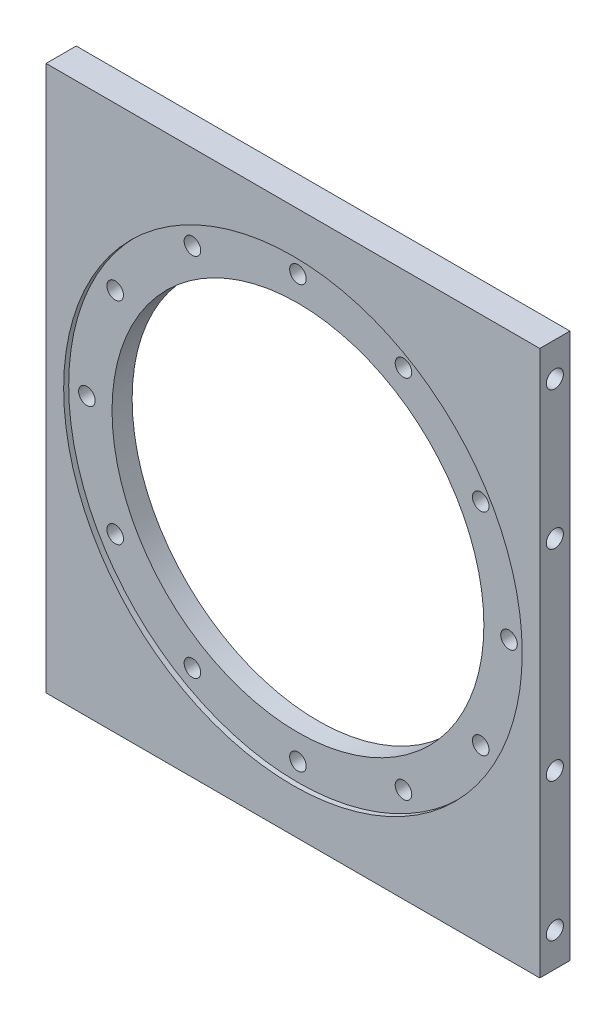
SolidWorks part; units mm, degrees
material "Q235A"
ref_plane "前视基准面" through (0, 0, 0) normal (0, 0, 1) x (1, 0, 0)
ref_plane "上视基准面" through (0, 0, 0) normal (0, 1, 0) x (1, 0, 0)
ref_plane "右视基准面" through (0, 0, 0) normal (1, 0, 0) x (0, 0, -1)
sketch "草图1" plane through (0, 0, 0) normal (0, 0, 1) x (1, 0, 0)
  line L1 (-98.25, -108.5) -> (98.25, -108.5)
  line L2 (-98.25, -108.5) -> (-98.25, 108.5)
  line L3 (-98.25, 108.5) -> (98.25, 108.5)
  line L4 (98.25, -108.5) -> (98.25, 108.5)
  line L5 (-98.25, -108.5) -> (98.25, 108.5) construction
  line L6 (-98.25, 108.5) -> (98.25, -108.5) construction
  circle A0 centre (0, 0) radius 74
  point P0 (0, 0)
  dimension "D3" = 148
  dimension "D1" = 196.5
  dimension "D2" = 217
extrude "凸台-拉伸1" add sketch "草图1" along normal blind 12
sketch "草图2" plane through (0, 0, 0) normal (0, 0, -1) x (-1, 0, 0)
  circle A0 centre (0, 0) radius 91.25
  dimension "D1" = 182.5
extrude "切除-拉伸1" cut sketch "草图2" against normal blind 2
sketch "草图3" plane through (0, 0, 12) normal (0, 0, 1) x (1, 0, 0)
  circle A1 centre (0, 0) radius 91.25
  circle A2 centre (0, 0) radius 91.25
  dimension "D1" = 0
extrude "切除-拉伸2" cut sketch "草图3" against normal blind 2
hole_wizard "M6 间隙孔1" positions "草图4" profile "草图5" hole size "M6" standard "ISO" end condition through all
sketch "草图4" plane through (0, 0, 10) normal (0, 0, 1) x (1, 0, 0)
  line L0 (0, 0) -> (0, 84) construction
  point P0 (0, 84)
  point P11 (42, 72.7461)
  point P12 (72.7461, 42)
  point P13 (84, 0)
  point P14 (72.7461, -42)
  point P15 (42, -72.7461)
  point P16 (0, -84)
  point P17 (-42, -72.7461)
  point P18 (-72.7461, -42)
  point P19 (-84, 0)
  point P20 (-72.7461, 42)
  point P21 (-42, 72.7461)
  point P24 (-1.3512, 0)
  point P25 (0, 0)
  dimension "D2" = 84
  dimension "D1" = 12
sketch "草图5" plane through (0, 84, 10) normal (1, 0, 0) x (0, -1, 0)
  line L0 (0, 0) -> (0, 10)
  line L1 (0, 10) -> (3.3, 10)
  line L2 (3.3, 10) -> (3.3, 0)
  line L5 (3.3, 0) -> (0, 0)
  line L11 (0, -6.35) -> (0, 107.95) construction
  dimension "通孔孔直径" = 6.6
  dimension "通孔孔深度" = 10
hole_wizard "M8 螺纹孔1" positions "草图6" profile "草图7" tap size "M8" standard "ISO"
sketch "草图6" plane through (-98.25, 0, 0) normal (-1, 0, 0) x (0, 0, 1)
  line L0 (0, 0) -> (12, 0) construction
  line L1 (12, 108.5) -> (12, -108.5) construction
  line L3 (6, 108.5) -> (6, 0) construction
  line L4 (12, 108.5) -> (0, 108.5) construction
  point P0 (6, 95)
  point P2 (6, 40)
  point P12 (6, -40)
  point P13 (6, -95)
  point P20 (6, 94.7928)
  dimension "D1" = 190
  dimension "D2" = 80
sketch "草图7" plane through (-98.25, 95, 6) normal (0, 1, 0) x (0, 0, 1)
  line L0 (0, 0) -> (0, 21.7929)
  line L1 (0, 21.7929) -> (3.4, 19.75)
  line L2 (3.4, 19.75) -> (3.4, 0)
  line L5 (3.4, 0) -> (0, 0)
  line L10 (0, 21.7929) -> (-3.4, 19.75) construction
  line L11 (0, -6.35) -> (0, 107.95) construction
  dimension "螺纹孔钻头直径" = 6.8
  dimension "螺纹孔钻头深度" = 19.75
  dimension "导头角度" = 118
hole_wizard "M8 螺纹孔2" positions "草图8" profile "草图9" tap size "M8" standard "ISO"
sketch "草图8" plane through (98.25, 0, 0) normal (1, 0, 0) x (0, 0, -1)
  point P0 (-6, 95)
  point P3 (-6, 40)
  point P6 (-6, -40)
  point P9 (-6, -95)
sketch "草图9" plane through (98.25, 95, 6) normal (0, 1, 0) x (0, 0, -1)
  line L0 (0, 0) -> (0, 21.7929)
  line L1 (0, 21.7929) -> (3.4, 19.75)
  line L2 (3.4, 19.75) -> (3.4, 0)
  line L5 (3.4, 0) -> (0, 0)
  line L10 (0, 21.7929) -> (-3.4, 19.75) construction
  line L11 (0, -6.35) -> (0, 107.95) construction
  dimension "螺纹孔钻头直径" = 6.8
  dimension "螺纹孔钻头深度" = 19.75
  dimension "导头角度" = 118
